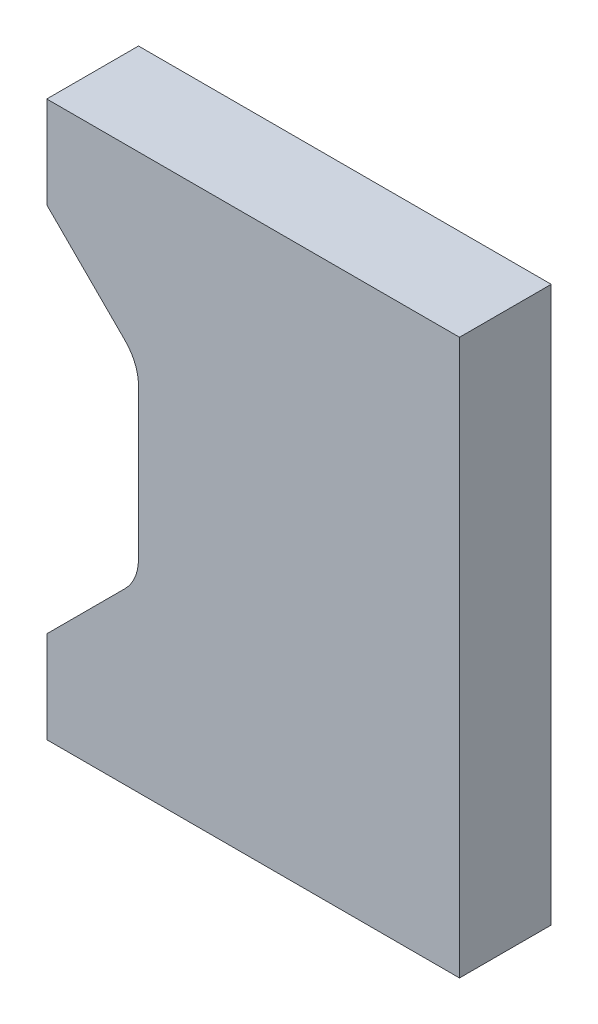
SolidWorks part; units mm, degrees
ref_plane "Front Plane" through (0, 0, 0) normal (0, 0, 1) x (1, 0, 0)
ref_plane "Top Plane" through (0, 0, 0) normal (0, 1, 0) x (1, 0, 0)
ref_plane "Right Plane" through (0, 0, 0) normal (1, 0, 0) x (0, 0, -1)
sketch "Sketch1" plane through (0, 0, 0) normal (0, 0, 1) x (1, 0, 0)
  line L0 (0, 0) -> (90, 0)
  line L1 (90, 0) -> (90, -121)
  line L2 (90, -121) -> (0, -121)
  line L3 (0, -121) -> (0, -101)
  line L4 (0, -101) -> (17.0711, -83.9289)
  line L5 (20, -76.8579) -> (20, -44.1421)
  line L6 (17.0711, -37.0711) -> (0, -20)
  line L7 (0, -20) -> (0, 0)
  arc A0 (17.0711, -83.9289) -> (20, -76.8579) centre (10, -76.8579) ccw
  arc A1 (20, -44.1421) -> (17.0711, -37.0711) centre (10, -44.1421) ccw
  dimension "D8" = 10
  dimension "D1" = 90
  dimension "D2" = 121
  dimension "D3" = 20
  dimension "D4" = 20
  dimension "D5" = 45
  dimension "D6" = 45
  dimension "D7" = 20
extrude "Boss-Extrude1" add sketch "Sketch1" along normal blind 20
